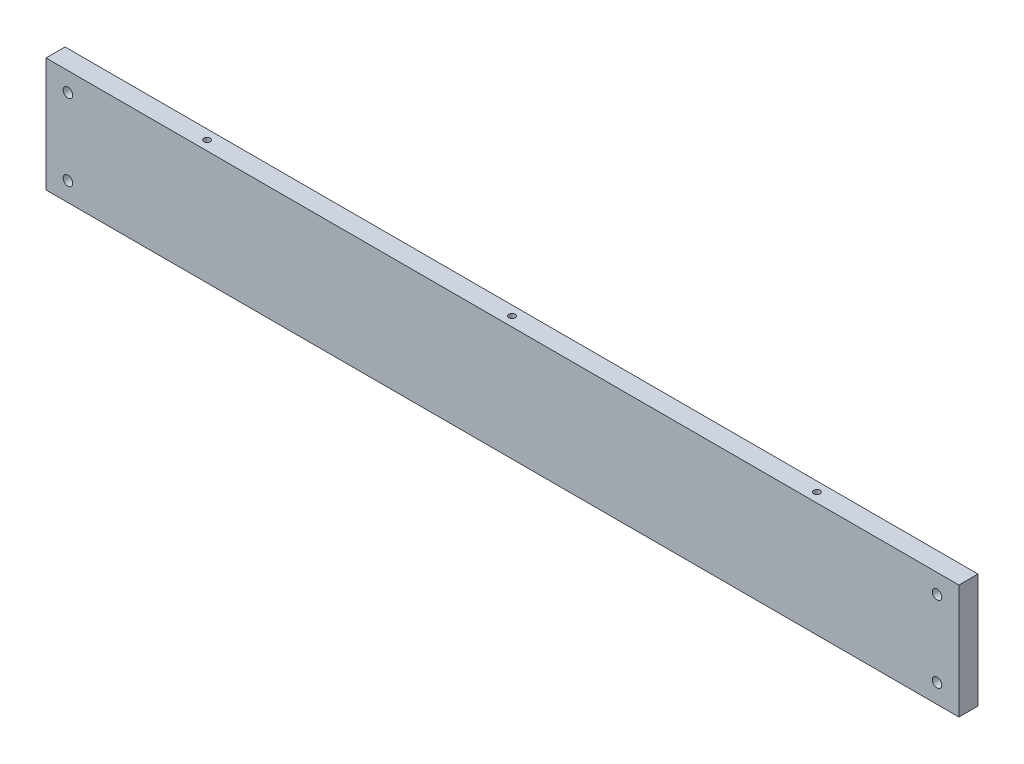
SolidWorks part; units mm, degrees
material "6061Al"
ref_plane "前视基准面" through (0, 0, 0) normal (0, 0, 1) x (1, 0, 0)
ref_plane "上视基准面" through (0, 0, 0) normal (0, 1, 0) x (1, 0, 0)
ref_plane "右视基准面" through (0, 0, 0) normal (1, 0, 0) x (0, 0, -1)
sketch "草图1" plane through (0, 0, 0) normal (0, 1, 0) x (1, 0, 0)
  line L1 (-239.5, -5) -> (239.5, -5)
  line L2 (-239.5, -5) -> (-239.5, 5)
  line L3 (-239.5, 5) -> (239.5, 5)
  line L4 (239.5, -5) -> (239.5, 5)
  line L5 (-239.5, -5) -> (239.5, 5) construction
  line L6 (-239.5, 5) -> (239.5, -5) construction
  point P0 (0, 0)
  dimension "D1" = 479
  dimension "D2" = 10
extrude "凸台-拉伸1" add sketch "草图1" along normal blind 60
hole_wizard "M5 螺纹孔1" positions "草图2" profile "草图3" tap size "M5" standard "ISO"
sketch "草图2" plane through (0, 0, 0) normal (0, -1, 0) x (-1, 0, 0)
  point P0 (0, 0)
  point P3 (-110, 0)
  point P6 (-220, 0)
  point P9 (220, 0)
  point P12 (110, 0)
sketch "草图3" plane through (0, 0, 0) normal (1, 0, 0) x (0, 0, -1)
  line L0 (0, 0) -> (0, 13.6618)
  line L1 (0, 13.6618) -> (2.1, 12.4)
  line L2 (2.1, 12.4) -> (2.1, 0)
  line L5 (2.1, 0) -> (0, 0)
  line L10 (0, 13.6618) -> (-2.1, 12.4) construction
  line L11 (0, -6.35) -> (0, 107.95) construction
  dimension "螺纹孔钻头直径" = 4.2
  dimension "螺纹孔钻头深度" = 12.4
  dimension "导头角度" = 118
cosmetic thread "孔螺蚊线1"
cosmetic thread "孔螺蚊线2"
cosmetic thread "孔螺蚊线3"
cosmetic thread "孔螺蚊线4"
cosmetic thread "孔螺蚊线5"
hole_wizard "M6 螺纹孔1" positions "草图4" profile "草图5" tap size "M6" standard "ISO" end condition through all
sketch "草图4" plane through (0, 0, -5) normal (0, 0, -1) x (-1, 0, 0)
  line L0 (0, 0) -> (0, 125.023) construction
  point P0 (228, 50)
  point P3 (228, 10)
  point P11 (-228, 10)
  point P12 (-228, 50)
sketch "草图5" plane through (-228, 50, -5) normal (1, 0, 0) x (0, 1, 0)
  line L0 (0, 0) -> (0, 10)
  line L1 (0, 10) -> (2.5, 10)
  line L2 (2.5, 10) -> (2.5, 0)
  line L5 (2.5, 0) -> (0, 0)
  line L11 (0, -6.35) -> (0, 107.95) construction
  dimension "通孔螺纹孔钻头直径" = 5
  dimension "通孔螺纹孔钻头深度" = 10
cosmetic thread "孔螺蚊线6"
cosmetic thread "孔螺蚊线7"
cosmetic thread "孔螺蚊线8"
cosmetic thread "孔螺蚊线9"
hole_wizard "M4 螺纹孔1" positions "草图6" profile "草图7" tap size "M4" standard "ISO"
sketch "草图6" plane through (0, 60, 0) normal (0, 1, 0) x (1, 0, 0)
  line L0 (0, 0) -> (0, 80.5996) construction
  point P0 (0, 0)
  point P3 (-160, 0)
  point P5 (160, 0)
  dimension "D1" = 320
sketch "草图7" plane through (0, 60, 0) normal (1, 0, 0) x (0, 0, 1)
  line L0 (0, 0) -> (0, 11.0914)
  line L1 (0, 11.0914) -> (1.65, 10.1)
  line L2 (1.65, 10.1) -> (1.65, 0)
  line L5 (1.65, 0) -> (0, 0)
  line L10 (0, 11.0914) -> (-1.65, 10.1) construction
  line L11 (0, -6.35) -> (0, 107.95) construction
  dimension "螺纹孔钻头直径" = 3.3
  dimension "螺纹孔钻头深度" = 10.1
  dimension "导头角度" = 118
cosmetic thread "孔螺蚊线10"
cosmetic thread "孔螺蚊线11"
cosmetic thread "孔螺蚊线12"
